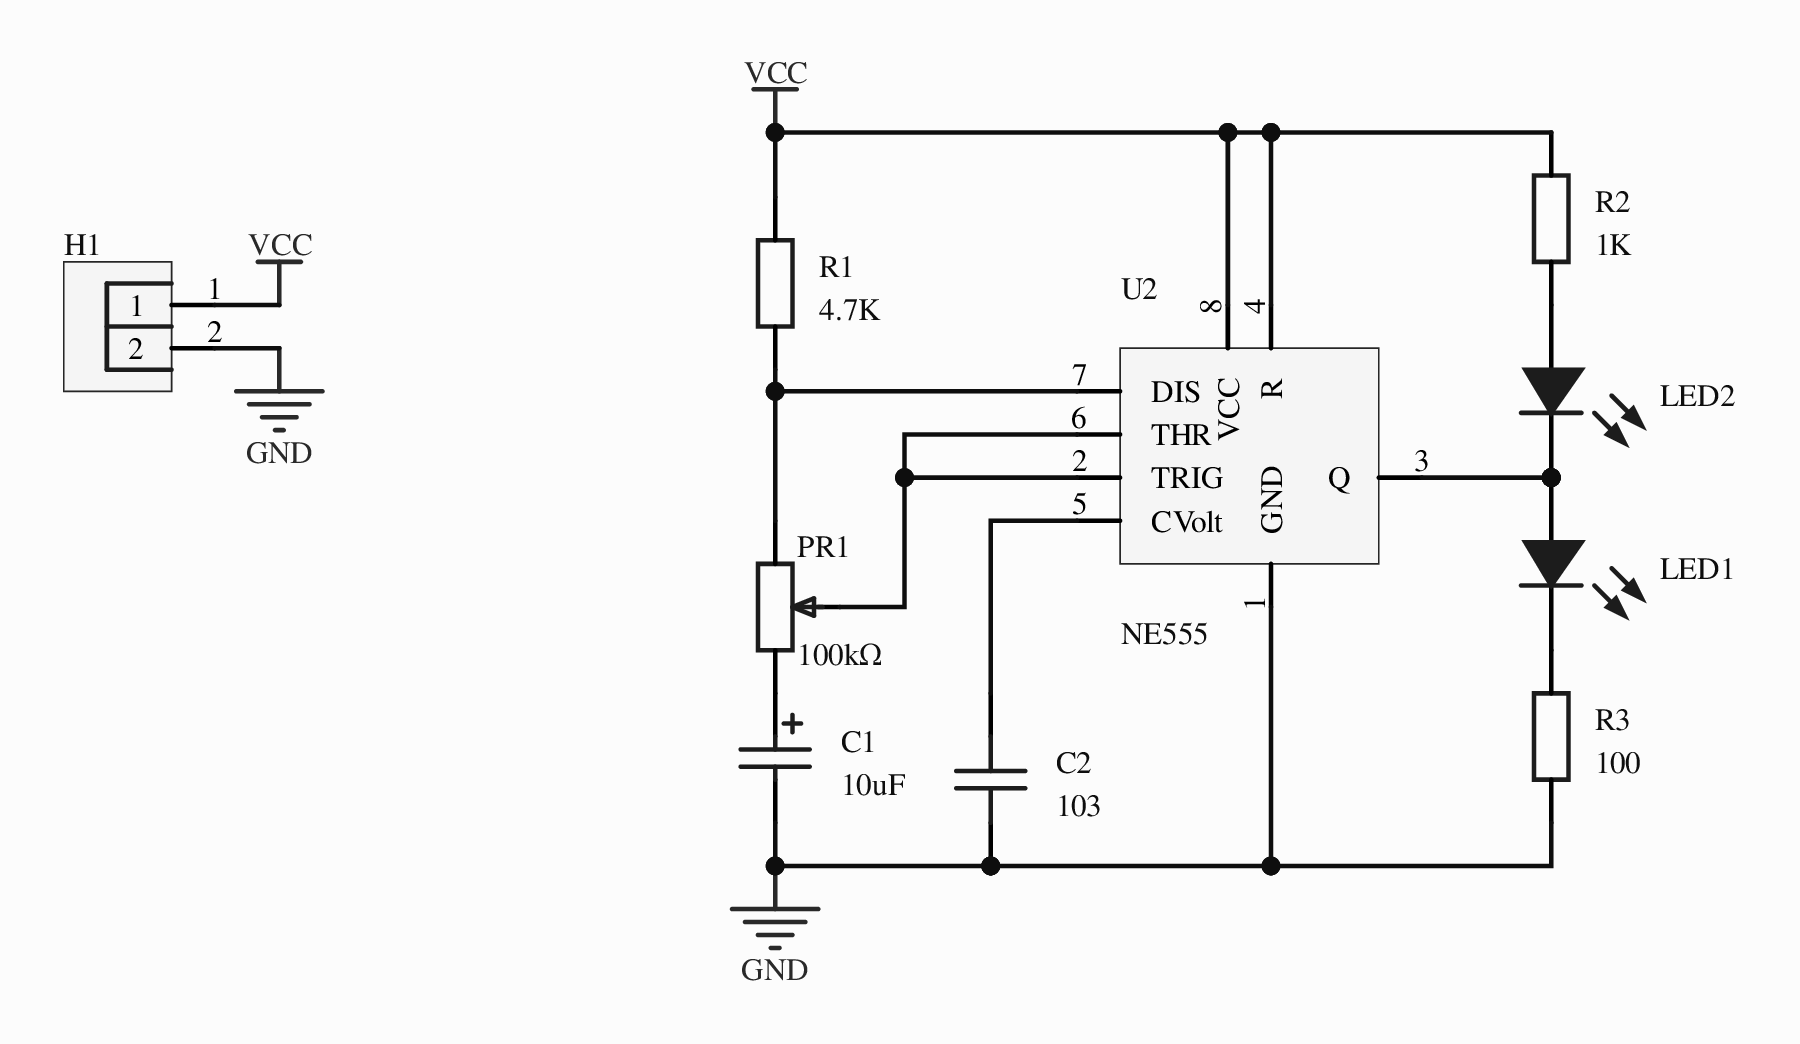
[diagram p0: MISC51886-3.schdoc]
# Altium project MISC51886-2.PrjPcb
1 sheet, 10 parts. Net scope: global (net labels, ports and power ports of the same name join across sheets).
Board file: MISC51886.pcbdoc

## Sheet MISC51886-3.schdoc
size 210 x 148 mm; Version: V1.0; @Project Name: MISC51886; @Update Date: 2026-10-07; @Create Date: 2026-10-07; @Board Name: MISC51886; @Create Time: 12:44:54; @Page Count: 1; @Page No: 1; @Schematic Name: MISC51886; @Update Time: 12:44:54; Size: A4

### Parts
C1  10uF  [C_Ele_SMD_3x5.4mm]
C2  103  [C0603]
H1  (no value)  [HDR-TH_2P-P2.54-V-M-1]
LED1  (no value)  [LED_0603]
LED2  (no value)  [LED_0603]
PR1  100kΩ  [R_3296]
R1  4.7K  [R0603]
R2  1K  [R0603]
R3  100  [R0603]
U2  NE555  [DIP-8_L9.8-W6.4-P2.54-LS7.6-BL]

### Nets
GND: C1.2 C2.1 H1.2 R3.1 U2.1(GND)
VCC: H1.1 R1.2 R2.2 U2.4(R) U2.8(VCC)
NetC1_1: C1.1 PR1.1
NetC2_2: C2.2 U2.5(CVolt)
NetLED1_1: LED1.1(C) R3.2
NetLED1_2: LED1.2(A) LED2.1(C) U2.3(Q)
NetLED2_2: LED2.2(A) R2.1
NetPR1_2: PR1.2 U2.2(TRIG) U2.6(THR)
NetPR1_3: PR1.3 R1.1 U2.7(DIS)

### Library data of the parts
C1 = C_Ele_SMD_3x5.4mm: Symbol: CAP_OLD; AddInBom: yes; ModelId: 0132c3d3fdbf4fd987f710a97e7a5b5d0819f05c4eef4c71ace90d822a990e87; ModelName: CAP-SMD_BD3.0-L3.3-W3.3-H5.3; ModelTransform: 129.9,149.58,209.06,-90,0,0,0,0,0; Device: C_Ele_SMD_3x5.4mm; FootprintName: C_Ele_SMD_3x5.4mm; Supplier Footprint: SMD,3x5.4mm; ConvertToPcb: yes; Value: 10uF
C2 = CAP_0603: Symbol: Capacitance; ConvertToPcb: yes; ModelId: ac125912035d415993ca9572d50418b10819f05c4eef4c71ace90d822a990e87; ModelName: C0603_L1.6-W0.8-H0.8; ModelTransform: 62.992,31.496,0,0,0,0,0,0,0; Device: CAP_0603; Value: 103; FootprintName: C0603; AddInBom: yes; Supplier Footprint: 0603
H1 = HDR-M_2.54_1x2P: Symbol: 210S-1*2P L=11.6MMGold-plated black; 3D Model: 79b2e9f2d70a4d68a1b7098f27c6d4c50819f05c4eef4c71ace90d822a990e87; 3D Model Transform: 200,100,0,0,0,0,0,0,-118.11; ConvertToPcb: yes; ModelName: HDR-M-2.54_1x2; Device: HDR-M_2.54_1x2P; Supplier Part: C124375; Supplier Footprint: 插件; FootprintName: HDR-TH_2P-P2.54-V-M-1; AddInBom: yes
LED1 LED2 = LED_0603-B: Symbol: LED_B; Convert to PCB: yes; 3D Model: eb8d964598f24248affda46f619856c50819f05c4eef4c71ace90d822a990e87; 3D Model Transform: 63.1,31.6,23.7,0,0,0,0,0,0; ModelName: LED-0603_B; Device: LED_0603-B; Add into BOM: yes; Supplier Footprint: 0603; FootprintName: LED_0603
PR1 = R_3296: ConvertToPcb: yes; ModelId: b182808559bb43bda9e7de64b64134cb0819f05c4eef4c71ace90d822a990e87; ModelName: 3296W; ModelTransform: 373.98,188.96,590.49,180,0,0,0,0,-140; Symbol: R_3296; Device: R_3296; Value: 100kΩ; FootprintName: R_3296; AddInBom: yes; Supplier Footprint: 直插
R1-R3 = Res_0603: Symbol: 电阻; 3D Model: fc143cca1e79419f9cd78b61e9279f080819f05c4eef4c71ace90d822a990e87; 3D Model Transform: 31.8897,63.7794,0,90,0,0,0,0,0; ConvertToPcb: yes; Device: Res_0603; Supplier Footprint: 0603; FootprintName: R0603; AddInBom: yes; ModelName: R0603
  R1: Value: 4.7K
  R2: Value: 1K
  R3: Value: 100
U2 = NE555: Manufacturer: TI; ManufacturerPart: NE555DR; AddInBom: yes; Pin Type: IN; OriginFootprint: SOIC-8_L4.9-W3.9-P1.27-LS6.0-BL; Symbol: NE555; Device: NE555; FootprintName: DIP-8_L9.8-W6.4-P2.54-LS7.6-BL; ConvertToPcb: yes; Supplier: LCSC; image: C7593.jpg; SupplierPart: C7593; JLCPCB Part Class: Basic; NO_CONNECT: yes